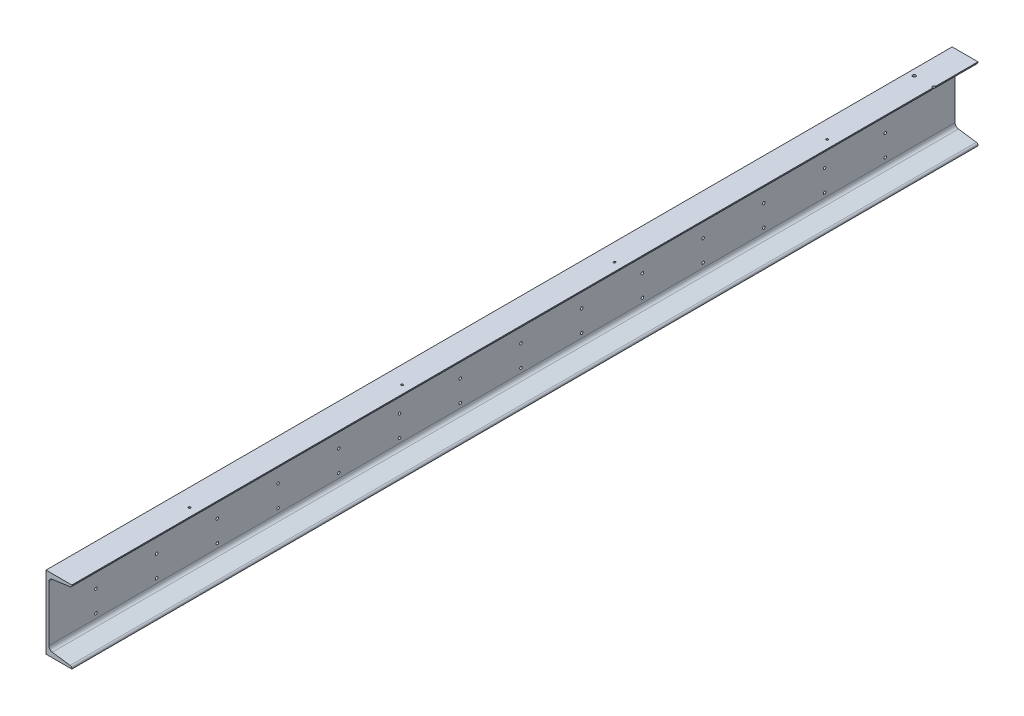
SolidWorks part; units mm, degrees
material "1023 碳钢板 (SS)"
ref_plane "前视基准面" through (0, 0, 0) normal (0, 0, 1) x (1, 0, 0)
ref_plane "上视基准面" through (0, 0, 0) normal (0, 1, 0) x (1, 0, 0)
ref_plane "右视基准面" through (0, 0, 0) normal (1, 0, 0) x (0, 0, -1)
sketch "草图1" plane through (0, 0, 0) normal (0, 0, 1) x (1, 0, 0)
  line L0 (0, 0) -> (-85, 0)
  line L1 (-85, 0) -> (-85, -240)
  line L2 (-85, -240) -> (0, -240)
  line L3 (0, -240) -> (0, -238.6233)
  line L4 (-5.5954, -232.1866) -> (-64.3093, -223.9349)
  line L5 (-75.5, -211.0614) -> (-75.5, -28.9386)
  line L6 (-64.3093, -16.0651) -> (-5.5954, -7.8134)
  line L7 (0, -1.3767) -> (0, 0)
  line L8 (-42.5, -227) -> (-42.5, -240) construction
  arc A0 (-64.3093, -223.9349) -> (-75.5, -211.0614) centre (-62.5, -211.0614) cw
  arc A1 (-75.5, -28.9386) -> (-64.3093, -16.0651) centre (-62.5, -28.9386) cw
  arc A2 (0, -238.6233) -> (-5.5954, -232.1866) centre (-6.5, -238.6233) ccw
  arc A3 (-5.5954, -7.8134) -> (0, -1.3767) centre (-6.5, -1.3767) ccw
  dimension "D7" = 13
  dimension "D8" = 6.5
  dimension "D1" = 240
  dimension "D2" = 85
  dimension "D3" = 42.5
  dimension "D4" = 13
  dimension "D5" = 9.5
  dimension "D6" = 8
extrude "凸台-拉伸1" add sketch "草图1" along normal blind 2985 contours A3 L6 A1 L5 A0 L4 A2 L3 L2 L1 L0 L7
sketch "草图2" plane through (-85, 0, 0) normal (-1, 0, 0) x (0, 0, 1)
  line L0 (2985, 0) -> (0, 0) construction
  line L1 (2985, 0) -> (2985, -240) construction
  circle A0 centre (2830, -126) radius 10
  circle A1 centre (2830, -196) radius 10
  circle A2 centre (2630, -126) radius 10
  circle A3 centre (2630, -196) radius 10
  circle A4 centre (2430, -126) radius 10
  circle A5 centre (2430, -196) radius 10
  circle A6 centre (2230, -126) radius 10
  circle A7 centre (2230, -196) radius 10
  circle A8 centre (2030, -126) radius 10
  circle A9 centre (2030, -196) radius 10
  circle A10 centre (1830, -126) radius 10
  circle A11 centre (1830, -196) radius 10
  circle A12 centre (1630, -126) radius 10
  circle A13 centre (1630, -196) radius 10
  circle A14 centre (1430, -126) radius 10
  circle A15 centre (1430, -196) radius 10
  circle A16 centre (1230, -126) radius 10
  circle A17 centre (1230, -196) radius 10
  circle A18 centre (1030, -126) radius 10
  circle A19 centre (1030, -196) radius 10
  circle A20 centre (830, -126) radius 10
  circle A21 centre (830, -196) radius 10
  circle A22 centre (630, -126) radius 10
  circle A23 centre (630, -196) radius 10
  circle A24 centre (430, -126) radius 10
  circle A25 centre (430, -196) radius 10
  circle A26 centre (230, -126) radius 10
  circle A27 centre (230, -196) radius 10
  dimension "D3" = 155
  dimension "D4" = 20
  dimension "D1" = 70
  dimension "D2" = 126
  dimension "D5" = 14
hole_wizard "M10 螺纹孔2" positions "草图5" profile "草图6" tap size "M10" standard "ISO"
sketch "草图5" plane through (-85, 0, 0) normal (-1, 0, 0) x (0, 0, 1)
  point P0 (230, -126)
  point P3 (230, -196)
  point P6 (430, -126)
  point P9 (430, -196)
  point P12 (630, -126)
  point P15 (630, -196)
  point P18 (830, -126)
  point P21 (830, -196)
  point P24 (1030, -126)
  point P27 (1030, -196)
  point P30 (1230, -126)
  point P33 (1230, -196)
  point P36 (1430, -126)
  point P39 (1430, -196)
  point P42 (1630, -196)
  point P45 (1630, -126)
  point P48 (1830, -196)
  point P51 (1830, -126)
  point P54 (2030, -126)
  point P57 (2030, -196)
  point P60 (2230, -196)
  point P63 (2230, -126)
  point P66 (2430, -126)
  point P69 (2430, -196)
  point P72 (2630, -196)
  point P75 (2630, -126)
  point P78 (2830, -126)
  point P81 (2830, -196)
sketch "草图6" plane through (-85, -126, 230) normal (0, 1, 0) x (0, 0, 1)
  line L0 (0, 0) -> (0, 27.0537)
  line L1 (0, 27.0537) -> (4.25, 24.5)
  line L2 (4.25, 24.5) -> (4.25, 0)
  line L5 (4.25, 0) -> (0, 0)
  line L10 (0, 27.0537) -> (-4.25, 24.5) construction
  line L11 (0, -6.35) -> (0, 107.95) construction
  dimension "螺纹孔钻头直径" = 8.5
  dimension "螺纹孔钻头深度" = 24.5
  dimension "导头角度" = 118
cosmetic thread "孔螺蚊线29" parameters "D1"=20, "D2"=10
cosmetic thread "孔螺蚊线30" parameters "D1"=20, "D2"=10
cosmetic thread "孔螺蚊线31" parameters "D1"=20, "D2"=10
cosmetic thread "孔螺蚊线32" parameters "D1"=20, "D2"=10
cosmetic thread "孔螺蚊线33" parameters "D1"=20, "D2"=10
cosmetic thread "孔螺蚊线34" parameters "D1"=20, "D2"=10
cosmetic thread "孔螺蚊线35" parameters "D1"=20, "D2"=10
cosmetic thread "孔螺蚊线36" parameters "D1"=20, "D2"=10
cosmetic thread "孔螺蚊线37" parameters "D1"=20, "D2"=10
cosmetic thread "孔螺蚊线38" parameters "D1"=20, "D2"=10
cosmetic thread "孔螺蚊线39" parameters "D1"=20, "D2"=10
cosmetic thread "孔螺蚊线40" parameters "D1"=20, "D2"=10
cosmetic thread "孔螺蚊线41" parameters "D1"=20, "D2"=10
cosmetic thread "孔螺蚊线42" parameters "D1"=20, "D2"=10
cosmetic thread "孔螺蚊线43" parameters "D1"=20, "D2"=10
cosmetic thread "孔螺蚊线44" parameters "D1"=20, "D2"=10
cosmetic thread "孔螺蚊线45" parameters "D1"=20, "D2"=10
cosmetic thread "孔螺蚊线46" parameters "D1"=20, "D2"=10
cosmetic thread "孔螺蚊线47" parameters "D1"=20, "D2"=10
cosmetic thread "孔螺蚊线48" parameters "D1"=20, "D2"=10
cosmetic thread "孔螺蚊线49" parameters "D1"=20, "D2"=10
cosmetic thread "孔螺蚊线50" parameters "D1"=20, "D2"=10
cosmetic thread "孔螺蚊线51" parameters "D1"=20, "D2"=10
cosmetic thread "孔螺蚊线52" parameters "D1"=20, "D2"=10
cosmetic thread "孔螺蚊线53" parameters "D1"=20, "D2"=10
cosmetic thread "孔螺蚊线54" parameters "D1"=20, "D2"=10
cosmetic thread "孔螺蚊线55" parameters "D1"=20, "D2"=10
cosmetic thread "孔螺蚊线56" parameters "D1"=20, "D2"=10
sketch "草图7" plane through (0, 0, 0) normal (0, 1, 0) x (1, 0, 0)
  line L0 (0, -2985) -> (-85, -2985) construction
  line L1 (0, -2985) -> (0, 0) construction
  circle A0 centre (-27, -470) radius 27.6787
  circle A1 centre (-27, -1170) radius 28.0203
  circle A2 centre (-27, -1870) radius 64.0719
  circle A3 centre (-27, -2570) radius 76.7633
  dimension "D6" = 55.3574
  dimension "D1" = 415
  dimension "D2" = 1115
  dimension "D3" = 1815
  dimension "D4" = 2515
  dimension "D5" = 27
hole_wizard "M8 螺纹孔1" positions "草图8" profile "草图9" tap size "M8" standard "ISO"
sketch "草图8" plane through (0, 0, 0) normal (0, 1, 0) x (1, 0, 0)
  point P0 (-27, -470)
  point P3 (-27, -1170)
  point P6 (-27, -1870)
  point P9 (-27, -2570)
sketch "草图9" plane through (-27, 0, 470) normal (1, 0, 0) x (0, 0, 1)
  line L0 (0, 0) -> (0, 21.7929)
  line L1 (0, 21.7929) -> (3.4, 19.75)
  line L2 (3.4, 19.75) -> (3.4, 0)
  line L5 (3.4, 0) -> (0, 0)
  line L10 (0, 21.7929) -> (-3.4, 19.75) construction
  line L11 (0, -6.35) -> (0, 107.95) construction
  dimension "螺纹孔钻头直径" = 6.8
  dimension "螺纹孔钻头深度" = 19.75
  dimension "导头角度" = 118
cosmetic thread "孔螺蚊线57" parameters "D1"=16, "D2"=8
cosmetic thread "孔螺蚊线58" parameters "D1"=16, "D2"=8
cosmetic thread "孔螺蚊线59" parameters "D1"=16, "D2"=8
cosmetic thread "孔螺蚊线60" parameters "D1"=16, "D2"=8
sketch "草图10" plane through (0, 0, 0) normal (0, 1, 0) x (1, 0, 0)
  line L0 (-85, -2985) -> (-85, 0) construction
  line L2 (0, -2985) -> (-85, -2985) construction
  circle A0 centre (-65, -145) radius 7.004
  circle A1 centre (0, -145) radius 6.3431
  dimension "D3" = 2840
  dimension "D1" = 65
  dimension "D2" = 20
hole_wizard "M12 螺纹孔1" positions "草图11" profile "草图12" tap size "M12" standard "ISO"
sketch "草图11" plane through (0, 0, 0) normal (0, 1, 0) x (1, 0, 0)
  point P0 (-65, -145)
  point P3 (0, -145)
sketch "草图12" plane through (-65, 0, 145) normal (1, 0, 0) x (0, 0, 1)
  line L0 (0, 0) -> (0, 32.3144)
  line L1 (0, 32.3144) -> (5.1, 29.25)
  line L2 (5.1, 29.25) -> (5.1, 0)
  line L5 (5.1, 0) -> (0, 0)
  line L10 (0, 32.3144) -> (-5.1, 29.25) construction
  line L11 (0, -6.35) -> (0, 107.95) construction
  dimension "螺纹孔钻头直径" = 10.2
  dimension "螺纹孔钻头深度" = 29.25
  dimension "导头角度" = 118
cosmetic thread "孔螺蚊线61" parameters "D1"=24, "D2"=12
sketch "草图13" plane through (-85, 0, 0) normal (-1, 0, 0) x (0, 0, 1)
  line L0 (2985, 0) -> (0, 0) construction
  line L1 (2985, 0) -> (2985, -240) construction
  circle A0 centre (1385, -50) radius 22.5
  dimension "D1" = 45
  dimension "D2" = 50
  dimension "D3" = 1600
extrude "切除-拉伸1" cut sketch "草图13" against normal blind 10
sketch "草图15" plane through (-85, 0, 0) normal (-1, 0, 0) x (0, 0, 1)
  line L0 (2985, 0) -> (2985, -240) construction
  line L1 (2985, 0) -> (0, 0) construction
  circle A0 centre (1675, -50) radius 20.466
  circle A1 centre (2785, -50) radius 30.8112
  point P8 (0, 0)
  dimension "D3" = 50
  dimension "D1" = 1110
  dimension "D2" = 200
hole_wizard "M6 螺纹孔1" positions "草图16" profile "草图17" tap size "M6" standard "GB"
sketch "草图16" plane through (-85, 0, 0) normal (-1, 0, 0) x (0, 0, 1)
  point P0 (1675, -50)
  point P3 (2785, -50)
sketch "草图17" plane through (-85, -50, 1675) normal (0, 1, 0) x (0, 0, 1)
  line L0 (0, 0) -> (0, 16.5022)
  line L1 (0, 16.5022) -> (2.5, 15)
  line L2 (2.5, 15) -> (2.5, 0)
  line L5 (2.5, 0) -> (0, 0)
  line L10 (0, 16.5022) -> (-2.5, 15) construction
  line L11 (0, -6.35) -> (0, 107.95) construction
  dimension "螺纹孔钻头直径" = 5
  dimension "螺纹孔钻头深度" = 15
  dimension "导头角度" = 118
cosmetic thread "孔螺蚊线63" parameters "D1"=12, "D2"=6
cosmetic thread "孔螺蚊线64" parameters "D1"=12, "D2"=6
